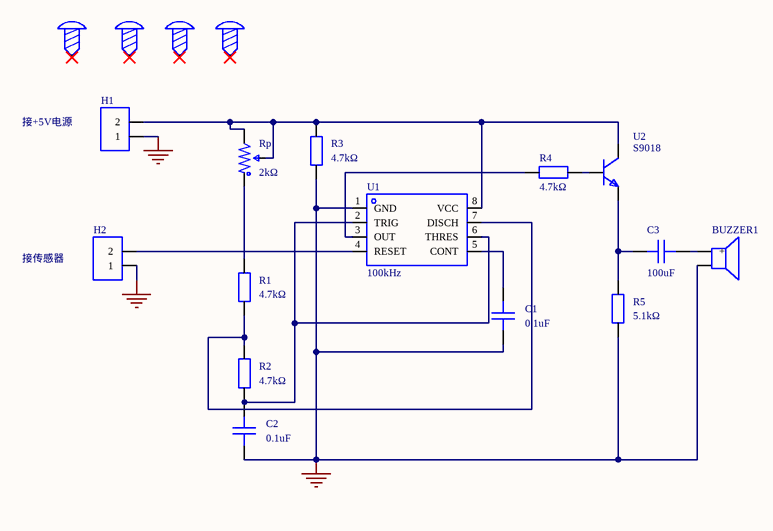
[diagram p0: MISC51754-3.schdoc]
# Altium project MISC51754-2.PrjPcb
1 sheet, 18 parts. Net scope: global (net labels, ports and power ports of the same name join across sheets).
Board file: MISC51754.pcbdoc

## Sheet MISC51754-3.schdoc
size 297 x 210 mm; Version: V1.0; @Project Name: MISC51754; @Page Count: 1; @Update Date: 2026-04-04; @Create Date: 2026-04-04; @Schematic Name: MISC51754; @Page No: 1; @Board Name: MISC51754; @Create Time: 17:18:05; @Update Time: 21:55:19

### Parts
BUZZER1  (no value)  [BUZ-TH_BD12.0-P7.60-D0.6-FD]
C1  0.1uF  [CAP-TH_L8.5-W5.0-P5.00-D1.2]
C2  0.1uF  [CAP-TH_L8.5-W5.0-P5.00-D1.2]
C3  100uF  [CAP-TH_L8.5-W5.0-P5.00-D1.2]
H1  (no value)  [HDR-TH_2P-P2.54-V-F]
H2  (no value)  [HDR-TH_2P-P2.54-V-F]
R1  4.7kΩ  [RES-TH_BD2.3-L6.5-P10.50-D0.5]
R2  4.7kΩ  [RES-TH_BD2.3-L6.5-P10.50-D0.5]
R3  4.7kΩ  [RES-TH_BD2.3-L6.5-P10.50-D0.5]
R4  4.7kΩ  [RES-TH_BD2.3-L6.5-P10.50-D0.5]
R5  5.1kΩ  [RES-TH_BD2.3-L6.5-P10.50-D0.5]
Rp  2kΩ  [RES-ADJ-TH_3P-L10.0-W10.0-P2.50-BL-BS]
SCREW1  (no value)  [M2螺丝]
SCREW2  (no value)  [M2螺丝]
SCREW3  (no value)  [M2螺丝]
SCREW4  (no value)  [M2螺丝]
U1  100kHz  [DIP-8_L9.8-W6.6-P2.54-LS7.6-BL]
U2  S9018  [TO-92-3_L4.8-W3.7-P1.27-L]

### Nets
GND: BUZZER1.2 C1.2 C2.1 H1.1 H2.1 R3.1 R5.1 U1.1(GND)
NetBUZZER1_1: BUZZER1.1(+) C3.1
NetC1_1: C1.1 U1.5(CONT)
NetC2_2: C2.2 R2.1 U1.2(TRIG) U1.6(THRES)
NetC3_2: C3.2 R5.2 U2.2(E)
NetH1_2: H1.2 R3.2 Rp.2 Rp.3 U1.8(VCC) U2.3(C)
NetH2_2: H2.2 U1.4(RESET)
NetR1_1: R1.1 R2.2 U1.7(DISCH)
NetR1_2: R1.2 Rp.1
NetR4_1: R4.1 U2.1(B)
NetR4_2: R4.2 U1.3(OUT)

Not connected (* = marked no-connect by the designer): SCREW1 1*; SCREW2 1*; SCREW3 1*; SCREW4 1*

### Notes on the sheet
- 接+5V电源
- 接传感器
- 2026-04-04
- 原理图
- P1
- 版本
- 尺寸
- A4
- 页
- 1
- 共

### Library data of the parts
BUZZER1 = TMB12A05_C96093: 驱动方式:有源(内含驱动线路);构造类型:电磁式;频率:2.7kHz;声压(SPL):85dB;; Manufacturer: 华能; AddInBom: yes; ModelId: 16ab50e14c5b4f2c986c135bdba60e37; ModelName: BUZ-TH_D12.0-H9.5-P7.60; ModelTransform: 472.44,472.176,0,90,0,0,-0.787,0,-177.165; Technology Type: 电磁式; Operating Voltage: 4V~8V; Sound Pressure Level (SPL): 85dB; Symbol: TMB12A05; Device: TMB12A05_C96093; LCSC Part Name: TMB12A05; ManufacturerPart: TMB12A05; Supplier Footprint: 插件,D=12mm; JLCPCB Part Class: 扩展库; Datasheet: https://atta.szlcsc.com/upload/public/pdf/source/20230426/A4FC10532558AA232D532AB83455FBA4.pdf; Supplier: LCSC; ConvertToPcb: yes; FootprintName: BUZ-TH_BD12.0-P7.60-D0.6-FD; Oscillator Circuit: 有源(内含驱动线路); Current Consumption: -; Diameter (φD): 12mm; Length: -; Width: -; Height: 9.8mm; Operating Temperature: -
C1-C3 = CT4-0805B104K500F3: 容值:100nF;精度:±10%;额定电压:50V;温度系数:X7R;; Manufacturer: FH(风华); AddInBom: yes; ModelId: 5610b656e7164072960d9d2d8c7d4fdf; ModelName: CAP-TH_L4.2-W3.8-H3.8-P5.08; ModelTransform: 222.8342,149.606,0,0,0,0,0,0,-118.11; Tolerance: ±10%; Voltage Rated: 50V; Temperature Coefficient: X7R; Symbol: CT4-0805B104K500F3; Device: CT4-0805B104K500F3; LCSC Part Name: 100nF ±10% 50V C3型（直脚）; ManufacturerPart: CT4-0805B104K500F3; Supplier Footprint: 插件,P=5.08mm; JLCPCB Part Class: 扩展库; Datasheet: https://atta.szlcsc.com/upload/public/pdf/source/20190402/C385200_059806A6312B28FF1421A2413EB641E1.pdf; Supplier: LCSC; ConvertToPcb: yes; FootprintName: CAP-TH_L8.5-W5.0-P5.00-D1.2
  C1 C2: Value: 0.1uF
  C3: Value: 100uF
H1 H2 = HDR-F_2.54_1x2P: Manufacturer: BOOMELE(博穆精密); Manufacturer Part: 2.54-1*2P母; Symbol: Header-Female-2.54_1x2; ConvertToPcb: yes; ModelId: a9450ef445564560a104363b9aacde4e; ModelName: HDR-TH_2P-P2.54-F-LI-1X2P; ModelTransform: 215.7476,98.425,0,0,0,0,0,0,-129.921; Device: HDR-F_2.54_1x2P; Supplier: LCSC; Supplier Part: C49661; JLCPCB Part Class: Extended Part; AddInBom: yes; Supplier Footprint: 插件; FootprintName: HDR-TH_2P-P2.54-V-F
R1-R5 = MF1/4W-4.7KΩ±1% T: 电阻类型:金属膜电阻;阻值:4.7kΩ;精度:±1%;功率:250mW;温度系数:±100ppm/℃;; Manufacturer: CCO(千志电子); Symbol: MF1/4W-4.7KΩ±1% T52; AddInBom: yes; ModelId: 8e6c7ee8323443d1ab8f0504b6353c8c; ModelName: RES-TH_D2.3-L6.5-P10.50; ModelTransform: 431.1015,91.3384,0,0,0,0,0.197,0,-137.795; Tolerance: ±1%; Overload Voltage (Max): 250V; Power(Watts): 250mW; Device: MF1/4W-4.7KΩ±1% T; LCSC Part Name: 4.7kΩ ±1% 250mW 金属膜电阻; ManufacturerPart: MF1/4W-4.7KΩ±1% T; Supplier Footprint: 插件,D2.3xL6.5mm; JLCPCB Part Class: 扩展库; Datasheet: https://atta.szlcsc.com/upload/public/pdf/source/20190910/C427326_62A6D058BC0FF74963A2F22379CA06CE.pdf; Supplier: LCSC; ConvertToPcb: yes; FootprintName: RES-TH_BD2.3-L6.5-P10.50-D0.5; Type: 金属膜电阻; Temperature Coefficient: ±100ppm/℃; Operating Temperature Range: -55℃~+155℃
  R1-R4: SupplierPart: C119339; Value: 4.7kΩ
  R5: Value: 5.1kΩ
Rp = 3296W-1-102: 阻值:1kΩ;精度:±10%;; Manufacturer: BOCHEN(博晨); AddInBom: yes; ModelId: b182808559bb43bda9e7de64b64134cb; ModelName: 3296W; ModelTransform: 374.015,188.976,0,90,0,0,0,0,-137.795; Tolerance: ±10%; Value: 2kΩ; Device: 3296W-1-102; Symbol: 3296W-1-102; LCSC Part Name: 1kΩ ±10%; ManufacturerPart: 3296W-1-102; Supplier Footprint: 插件; JLCPCB Part Class: 扩展库; Datasheet: https://atta.szlcsc.com/upload/public/pdf/source/20171114/C118949_15106326635991117438.pdf; Supplier: LCSC; ConvertToPcb: yes; FootprintName: RES-ADJ-TH_3P-L10.0-W10.0-P2.50-BL-BS
SCREW1-SCREW4 = M2螺丝: Symbol: 螺丝孔; ConvertToPcb: yes; Device: M2螺丝; AddInBom: yes; Supplier Footprint: 插件; FootprintName: M2螺丝
U1 = NE555P: 频率:100kHz;; Manufacturer: TI(德州仪器); AddInBom: yes; ModelId: db2af726fcec488f8bf8e467aca974b3; ModelName: DIP-8_L9.8-W6.6-H3.5-LS7.62-P2.54; ModelTransform: 385.826,311.8104,0,0,0,0,-1.693,0,-137.795; Supply Voltage: 4.5V~16V; Supply Current: 10mA; Device: NE555P; Symbol: NE555P; LCSC Part Name: NE555P; SupplierPart: C46749; ManufacturerPart: NE555P; Supplier Footprint: DIP-8; JLCPCB Part Class: 扩展库; Datasheet: https://www.ti.com/cn/lit/gpn/ne555; Supplier: LCSC; ConvertToPcb: yes; FootprintName: DIP-8_L9.8-W6.6-P2.54-LS7.6-BL; Value: 100kHz; Operating Temperature: 0℃~+70℃
U2 = MPSH10_C3197038: 晶体管类型:NPN;集电极电流(Ic):-;集射极击穿电压(Vceo):25V;功率(Pd):350mW;直流电流增益(hFE@Ic,Vce):60@4mA,10V;; Manufacturer: onsemi(安森美); AddInBom: yes; ModelId: e2f2caf48bbc414b83cacb7c7f8d5f8b; ModelTransform: 188.466,153.543,0,0,0,0,0,19.173,-118.11; Transistor Type: NPN; Collector-Emitter Breakdown Voltage (Vceo): 25V; Power Dissipation (Pd): 350mW; Transition Frequency (fT): 650MHz; Symbol: MPSH10_C3197038; Manufacturer Part: S9018; Device: MPSH10_C3197038; LCSC Part Name: NPN 耐压:25V; SupplierPart: C3197038; Supplier Footprint: 插件; JLCPCB Part Class: 扩展库; Datasheet: https://atta.szlcsc.com/upload/public/pdf/source/20230915/DE7375A4D892B19EEF6BFAE95203FBDB.pdf; Supplier: LCSC; ConvertToPcb: yes; FootprintName: TO-92-3_L4.8-W3.7-P1.27-L; ModelName: TO-92-3_L4.8-W3.7-P1.27-L; Collector Current (Ic): -; DC Current Gain (hFE@Ic,Vce): 60@4mA,10V; Operating Temperature: -65℃~+150℃@(Tj)